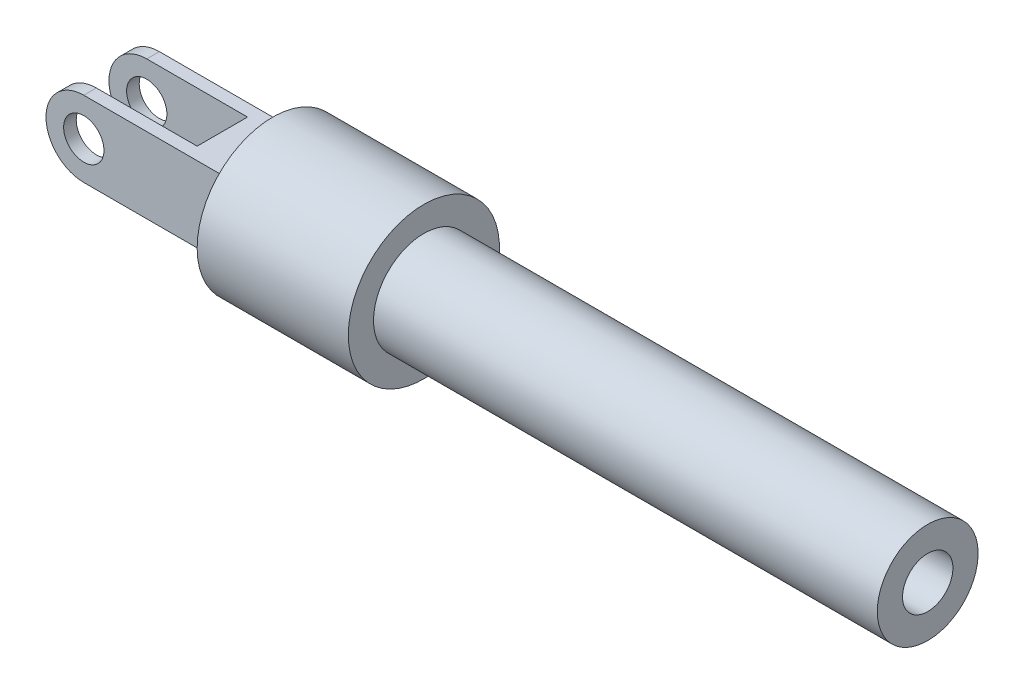
SolidWorks part; units mm, degrees
ref_plane "Front Plane" through (0, 0, 0) normal (0, 0, 1) x (1, 0, 0)
ref_plane "Top Plane" through (0, 0, 0) normal (0, 1, 0) x (1, 0, 0)
ref_plane "Right Plane" through (0, 0, 0) normal (1, 0, 0) x (0, 0, -1)
sketch "Sketch1" plane through (0, 0, 0) normal (0, 0, 1) x (1, 0, 0)
  line L0 (0, -60.0721) -> (0, 2943.5314) construction
  line L1 (0, 0) -> (0, 1.5)
  line L2 (0, 1.5) -> (3, 1.5)
  line L3 (3, 1.5) -> (3, 1)
  line L4 (3, 1) -> (13, 1)
  line L5 (13, 1) -> (13, 0)
  line L6 (0.1244, 0) -> (3003.7278, 0) construction
  line L7 (0, 0) -> (13, 0)
  point P8 (3, 1.25)
  dimension "D1" = 3
  dimension "D2" = 10
  dimension "D3" = 3
  dimension "D4" = 2
revolve "Revolve1" add sketch "Sketch1" angle 360 about L6
sketch "Sketch2" plane through (0, 0, 0) normal (0, 0, 1) x (1, 0, 0)
  line L0 (0, 0) -> (-50000, 0) construction
  line L1 (0, 0.75) -> (0, -0.75)
  line L2 (0, 1.5) -> (0, -1.5) construction
  line L3 (0, -0.75) -> (-3, -0.75)
  line L4 (0, 0) -> (0, 50000) construction
  line L5 (0, 0.75) -> (-3, 0.75)
  arc A0 (-3, -0.75) -> (-3, 0.75) centre (-3, 0) cw
  circle A1 centre (-3, 0) radius 0.4
  point P9 (0, 0)
  dimension "D1" = 0.75
  dimension "D3" = 0.8
  dimension "D2" = 3
extrude "Boss-Extrude1" add sketch "Sketch2" along normal mid plane 1.5
sketch "Sketch3" plane through (0, 0, 0) normal (0, 0, 1) x (1, 0, 0)
  line L0 (-1, 0.75) -> (-1, -0.75)
  line L1 (0, 0.75) -> (-3, 0.75) construction
  line L2 (-3, -0.75) -> (0, -0.75) construction
  line L3 (-1, -0.75) -> (-3, -0.75)
  line L4 (-3, 0.75) -> (-1, 0.75)
  line L5 (0, 1.5) -> (0, -1.5) construction
  arc A0 (-3, -0.75) -> (-3, 0.75) centre (-3, 0) cw
  dimension "D1" = 1
extrude "Cut-Extrude1" cut sketch "Sketch3" against normal mid plane 1
sketch "Sketch4" plane through (13, 0, 0) normal (1, 0, 0) x (0, 0, -1)
  circle A0 centre (0, 0) radius 0.5
extrude "Cut-Extrude2" cut sketch "Sketch4" against normal blind 6
